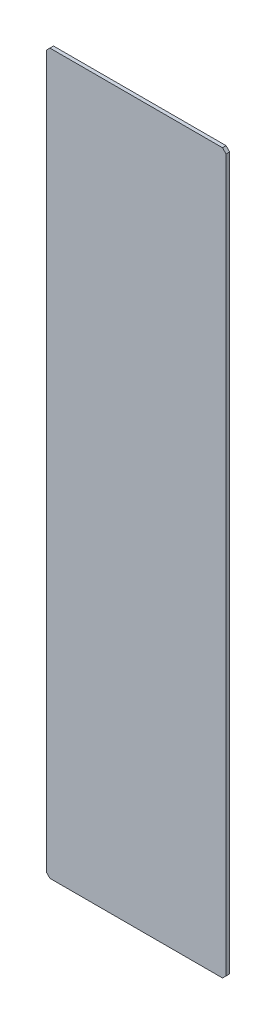
SolidWorks part; units mm, degrees
ref_plane "前视基准面" through (0, 0, 0) normal (0, 0, 1) x (1, 0, 0)
ref_plane "上视基准面" through (0, 0, 0) normal (0, 1, 0) x (1, 0, 0)
ref_plane "右视基准面" through (0, 0, 0) normal (1, 0, 0) x (0, 0, -1)
sketch "草图1" plane through (0, 0, 0) normal (0, 0, 1) x (1, 0, 0)
  line L1 (-250, -1000) -> (250, -1000)
  line L2 (-250, -1000) -> (-250, 1000)
  line L3 (-250, 1000) -> (250, 1000)
  line L4 (250, -1000) -> (250, 1000)
  line L5 (-250, -1000) -> (250, 1000) construction
  line L6 (-250, 1000) -> (250, -1000) construction
  point P0 (0, 0)
  dimension "D1" = 500
  dimension "D2" = 2000
extrude "凸台-拉伸1" add sketch "草图1" along normal mid plane 10
chamfer "倒角1" distance 10 angle 45 4 edges at (-250, 1000, 0) (-250, -1000, 0) (250, -1000, 0) (250, 1000, 0)
